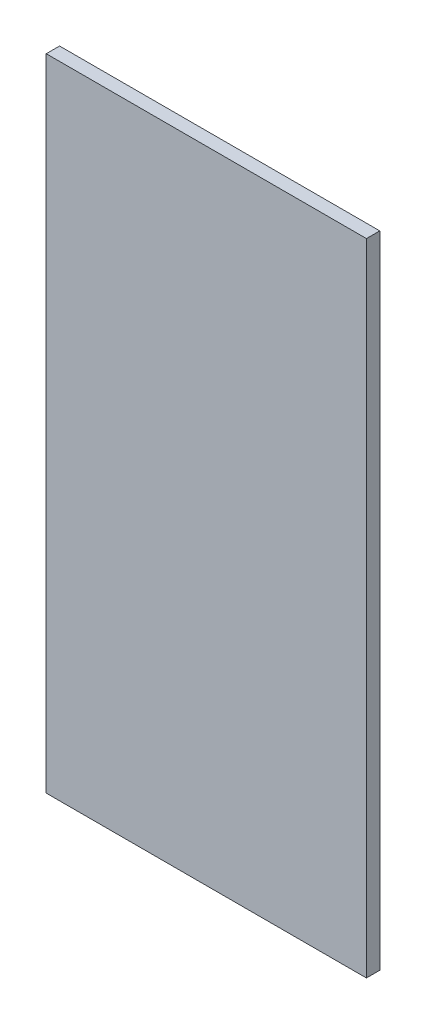
SolidWorks part; units mm, degrees
ref_plane "前视基准面" through (0, 0, 0) normal (0, 0, 1) x (1, 0, 0)
ref_plane "上视基准面" through (0, 0, 0) normal (0, 1, 0) x (1, 0, 0)
ref_plane "右视基准面" through (0, 0, 0) normal (1, 0, 0) x (0, 0, -1)
sketch "草图1" plane through (0, 0, 0) normal (0, 0, 1) x (1, 0, 0)
  line L0 (16.7448, 0) -> (16.7448, 240)
  line L1 (16.7448, 240) -> (136.7448, 240)
  line L2 (136.7448, 240) -> (136.7448, 0)
  line L3 (136.7448, 0) -> (16.7448, 0)
extrude "凸台-拉伸1" add sketch "草图1" along normal blind 5
